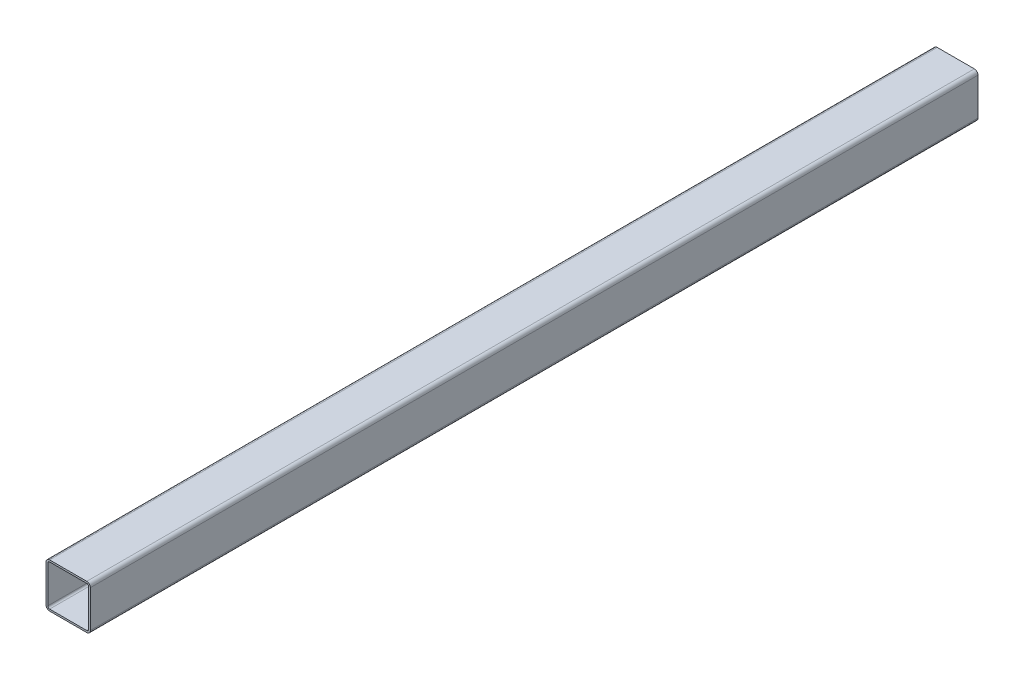
SolidWorks part; units mm, degrees
material "1023 碳钢板 (SS)"
ref_plane "Front Plane" through (0, 0, 0) normal (0, 0, 1) x (1, 0, 0)
ref_plane "Top Plane" through (0, 0, 0) normal (0, 1, 0) x (1, 0, 0)
ref_plane "Right Plane" through (0, 0, 0) normal (1, 0, 0) x (0, 0, -1)
sketch "Sketch1" plane through (0, 0, 0) normal (0, 0, 1) x (1, 0, 0)
  line L1 (41.8, 50) -> (-41.8, 50)
  line L2 (50, 41.8) -> (50, -41.8)
  line L3 (41.8, -50) -> (-41.8, -50)
  line L4 (-50, 41.8) -> (-50, -41.8)
  line L5 (50, 50) -> (-50, -50) construction
  line L6 (50, -50) -> (-50, 50) construction
  arc A0 (-41.8, -50) -> (-50, -41.8) centre (-41.8, -41.8) cw
  arc A1 (50, -41.8) -> (41.8, -50) centre (41.8, -41.8) cw
  arc A2 (41.8, 50) -> (50, 41.8) centre (41.8, 41.8) cw
  arc A3 (-50, 41.8) -> (-41.8, 50) centre (-41.8, 41.8) cw
  point P0 (0, 0)
  dimension "D3" = 8.2
  dimension "D1" = 100
  dimension "D2" = 100
extrude "Boss-Extrude1" add sketch "Sketch1" along normal blind 2000
shell "Shell1" thickness 4
